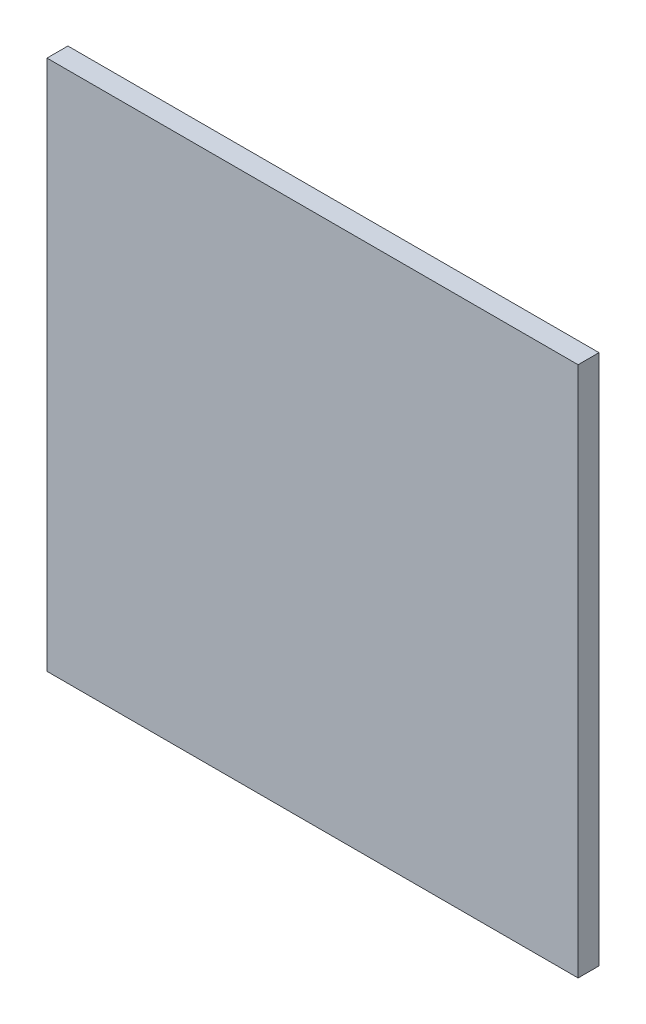
from build123d import *

# Parameters (mm, degrees)
SKETCH1_W           = 254
SKETCH1_H           = 254
BOSS_EXTRUDE1_DEPTH = 5


with BuildPart() as part:
    # Sketch1 → Boss-Extrude1 (new, symmetric)
    with BuildSketch(Plane.XY):
        Rectangle(SKETCH1_W, SKETCH1_H)
    extrude(amount=BOSS_EXTRUDE1_DEPTH, both=True)


solid = part.part
